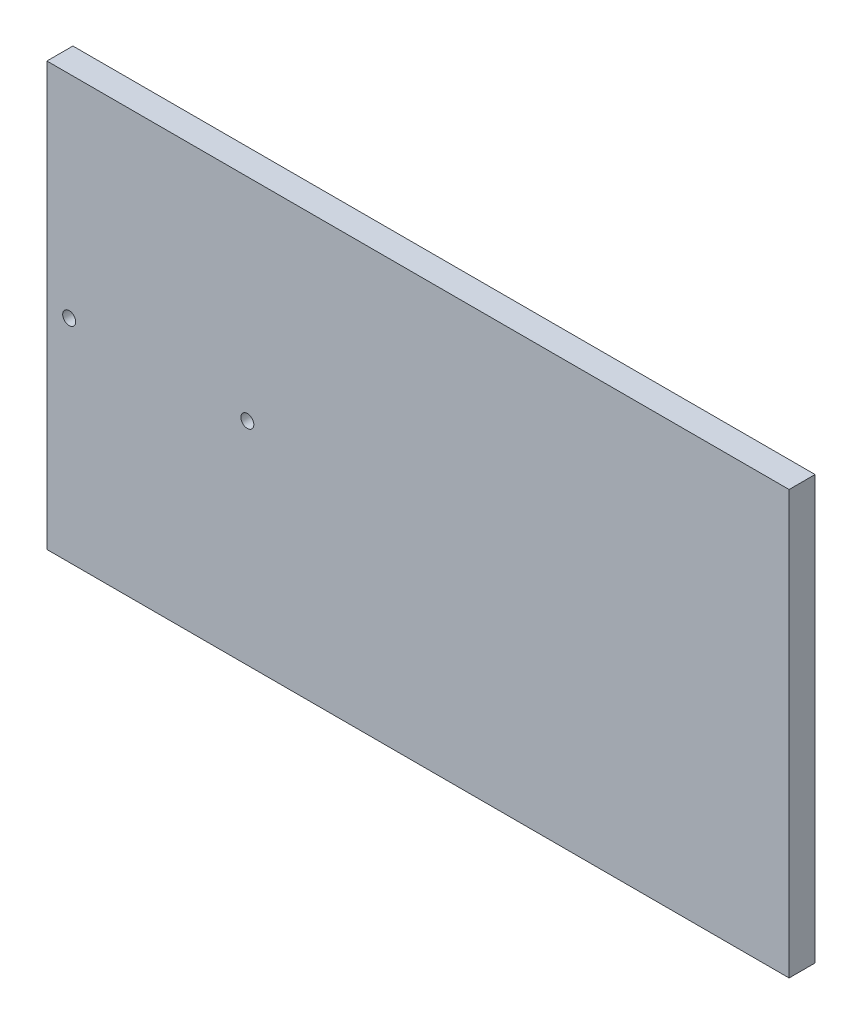
SolidWorks part; units mm, degrees
material "普通碳钢"
ref_plane "Front Plane" through (0, 0, 0) normal (0, 0, 1) x (1, 0, 0)
ref_plane "Top Plane" through (0, 0, 0) normal (0, 1, 0) x (1, 0, 0)
ref_plane "Right Plane" through (0, 0, 0) normal (1, 0, 0) x (0, 0, -1)
sketch "Sketch1" plane through (0, 0, 0) normal (0, 0, 1) x (1, 0, 0)
  line L0 (0, 0) -> (0, 570)
  line L1 (0, 570) -> (1000, 570)
  line L3 (0, 0) -> (1000, 0)
  line L5 (0, 285) -> (270, 285) construction
  line L6 (1000, 0) -> (1000, 570)
  dimension "D1" = 570
  dimension "D2" = 270
  dimension "D4" = 1000
extrude "Boss-Extrude1" add sketch "Sketch1" along normal blind 35
hole_wizard "M20 Tapped Hole1" positions "3DSketch1" profile "Sketch2" tap size "M20" standard "GB" end condition through all
sketch3d "3DSketch1"
  line L1 (0, 570, 35) -> (0, 0, 35) construction
  line L7 (0, 285, 35) -> (1000, 285, 35) construction
  line L8 (1000, 0, 35) -> (1000, 570, 35) construction
  point P0 (30, 285, 35)
  point P2 (270, 285, 35)
  dimension "D1" = 30
  dimension "D2" = 240
sketch "Sketch2" plane through (30, 285, 35) normal (1, 0, 0) x (0, -1, 0)
  line L0 (0, 0) -> (0, 35)
  line L1 (0, 35) -> (8.75, 35)
  line L2 (8.75, 35) -> (8.75, 0)
  line L5 (8.75, 0) -> (0, 0)
  line L11 (0, -6.35) -> (0, 107.95) construction
  dimension "通孔螺纹孔钻头直径" = 17.5
  dimension "通孔螺纹孔钻头深度" = 35
cosmetic thread "Tapped hole thread 1" parameters "D2"=20
cosmetic thread "Tapped hole thread 2" parameters "D2"=20
